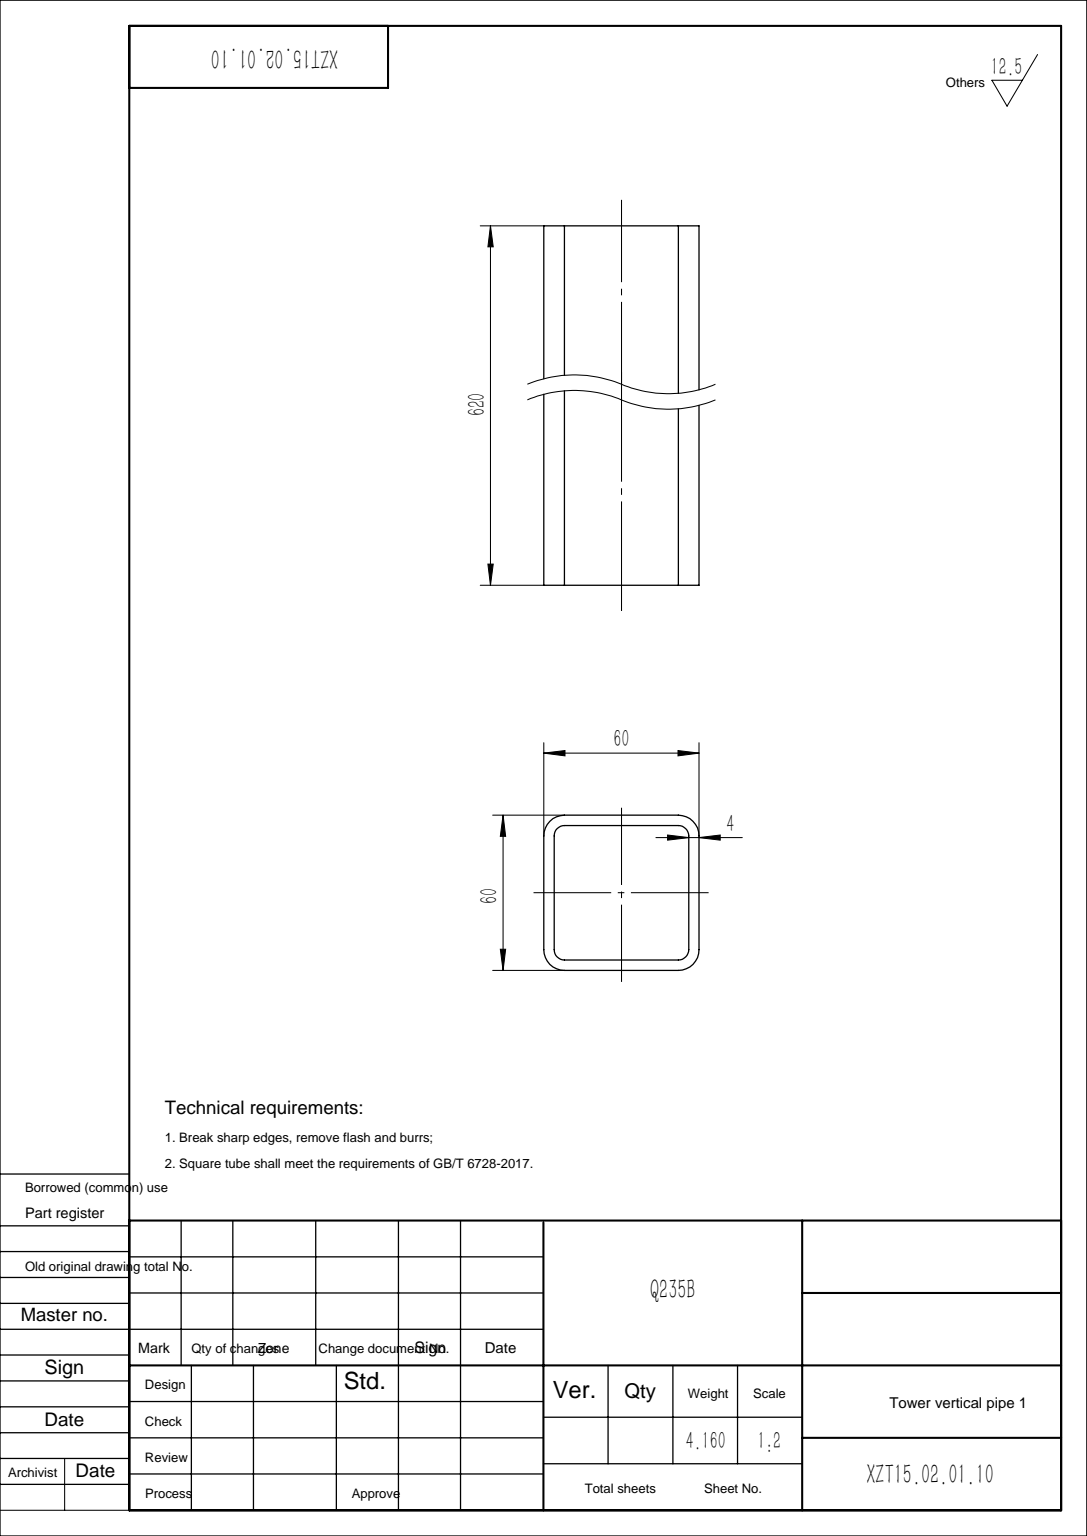
from build123d import *

# Parameters (mm, degrees)
GB_T_6728_2002_SQUARE_HOLLOW_SECTION_60_DEPTH = 620


with BuildPart() as part:
    # Sketch1 → GB/T 6728-2002 square hollow section 60×60×4(1) (new body)
    with BuildSketch(Plane(origin=(0, 0, 0), x_dir=(-1, 0, 0), z_dir=(0, 1, 0))):
        with BuildLine():
            Line((-22, -30), (22, -30))
            ThreePointArc((22, -30), (27.656854249, -27.656854249), (30, -22))
            Line((30, -22), (30, 22))
            ThreePointArc((30, 22), (27.656854249, 27.656854249), (22, 30))
            Line((22, 30), (-22, 30))
            ThreePointArc((-22, 30), (-27.656854249, 27.656854249), (-30, 22))
            Line((-30, 22), (-30, -22))
            ThreePointArc((-30, -22), (-27.656854249, -27.656854249), (-22, -30))
        make_face()
        with BuildLine():
            Line((-22, -26), (22, -26))
            ThreePointArc((22, -26), (24.828427125, -24.828427125), (26, -22))
            Line((26, -22), (26, 22))
            ThreePointArc((26, 22), (24.828427125, 24.828427125), (22, 26))
            Line((22, 26), (-22, 26))
            ThreePointArc((-22, 26), (-24.828427125, 24.828427125), (-26, 22))
            Line((-26, 22), (-26, -22))
            ThreePointArc((-26, -22), (-24.828427125, -24.828427125), (-22, -26))
        make_face(mode=Mode.SUBTRACT)
    extrude(amount=GB_T_6728_2002_SQUARE_HOLLOW_SECTION_60_DEPTH)


solid = part.part
